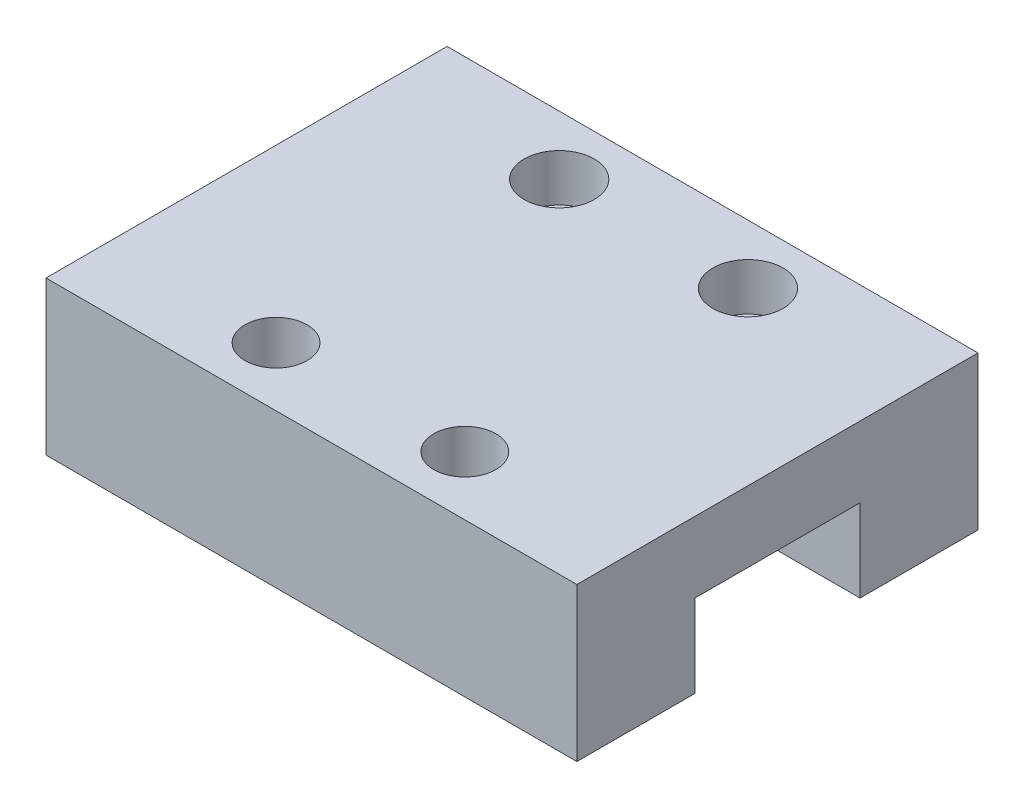
SolidWorks part; units mm, degrees
ref_plane "Front" through (0, 0, 0) normal (0, 0, 1) x (1, 0, 0)
ref_plane "Top" through (0, 0, 0) normal (0, 1, 0) x (1, 0, 0)
ref_plane "Right" through (0, 0, 0) normal (1, 0, 0) x (0, 0, -1)
sketch "Sketch1" plane through (0, 0, 0) normal (1, 0, 0) x (0, 0, -1)
  line L0 (0.2415, 5.0469) -> (0.2415, -2.9702) construction
  line L1 (-8.2585, 5.0469) -> (8.7415, 5.0469)
  line L2 (-8.2585, 5.0469) -> (-8.2585, -1.4531)
  line L3 (-8.2585, -1.4531) -> (-3.2585, -1.4531)
  line L4 (8.7415, 5.0469) -> (8.7415, -1.4531)
  line L5 (-3.2585, -1.4531) -> (-3.2585, 2.0469)
  line L6 (-3.2585, 2.0469) -> (3.7415, 2.0469)
  line L7 (3.7415, 2.0469) -> (3.7415, -1.4531)
  line L8 (3.7415, -1.4531) -> (8.7415, -1.4531)
  dimension "D1" = 17
  dimension "D2" = 6.5
  dimension "D3" = 7
  dimension "D4" = 3.5
  dimension "D5" = 3.5
extrude "Boss-Extrude1" add sketch "Sketch1" along normal mid plane 22.5
sketch "Sketch2" plane through (0, 5.0469, 0) normal (0, 1, 0) x (1, 0, 0)
  line L0 (0, 8.7415) -> (0, -10.6019) construction
  line L1 (11.25, 0.2415) -> (-11.25, 0.2415) construction
  line L2 (11.25, 8.7415) -> (11.25, -8.2585) construction
  line L3 (-11.25, 8.7415) -> (-11.25, -8.2585) construction
  line L4 (11.25, 8.7415) -> (-11.25, 8.7415) construction
  circle A0 centre (4, -5.7585) radius 1.3174
  circle A1 centre (-4, 6.2415) radius 1.4885
  circle A2 centre (4, 6.2415) radius 1.4885
  circle A3 centre (-4, -5.7585) radius 1.3174
  dimension "D1" = 6
  dimension "D2" = 6
  dimension "D3" = 8
  dimension "D4" = 4
  dimension "D5" = 4
  dimension "D6" = 4
  dimension "D7" = 4
extrude "Cut-Extrude1" cut sketch "Sketch2" against normal blind 2
